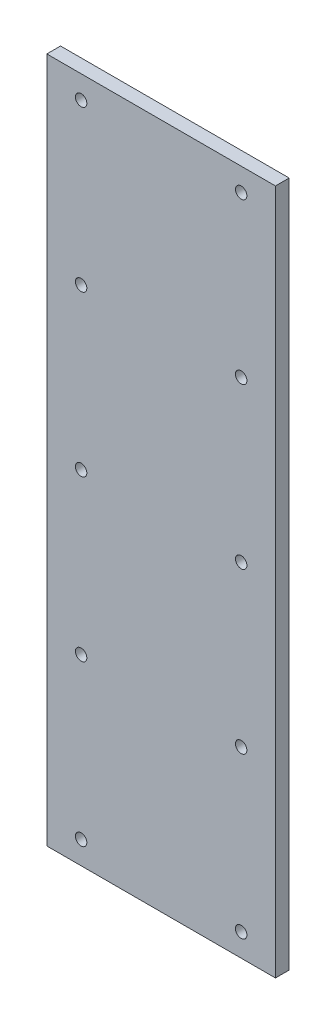
SolidWorks part; units mm, degrees
material "Q235B"
ref_plane "Front Plane" through (0, 0, 0) normal (0, 0, 1) x (1, 0, 0)
ref_plane "Top Plane" through (0, 0, 0) normal (0, 1, 0) x (1, 0, 0)
ref_plane "Right Plane" through (0, 0, 0) normal (1, 0, 0) x (0, 0, -1)
other "Configuration Table"
sketch "Sketch1" plane through (0, 0, 0) normal (0, 0, 1) x (1, 0, 0)
  line L1 (-50, -150) -> (50, -150)
  line L2 (-50, -150) -> (-50, 150)
  line L3 (-50, 150) -> (50, 150)
  line L4 (50, -150) -> (50, 150)
  line L5 (-50, -150) -> (50, 150) construction
  line L6 (-50, 150) -> (50, -150) construction
  circle A0 centre (-35, 0) radius 5.5 construction
  point P0 (0, 0)
  dimension "D1" = 100
  dimension "D2" = 300
  dimension "D3" = 0
  dimension "D4" = 35
extrude "Boss-Extrude1" add sketch "Sketch1" along normal blind 6
hole_wizard "M6 Tapped Hole1" positions "Sketch2" profile "Sketch4" tap size "M6" standard "GB" end condition through all
sketch "Sketch2" plane through (0, 0, 6) normal (0, 0, 1) x (1, 0, 0)
  point P0 (-35, 0)
sketch "Sketch4" plane through (-35, 0, 6) normal (1, 0, 0) x (0, -1, 0)
  line L0 (0, 0) -> (0, 6)
  line L1 (0, 6) -> (2.5, 6)
  line L2 (2.5, 6) -> (2.5, 0)
  line L5 (2.5, 0) -> (0, 0)
  line L11 (0, -6.35) -> (0, 107.95) construction
  dimension "通孔螺纹孔钻头直径" = 5
  dimension "通孔螺纹孔钻头深度" = 6
cosmetic thread "Cosmetic thread 1" parameters "D2"=6
pattern_linear "LPattern1" count 3 spacing 70 along (0, -1, 0) count 2 spacing 70 along (1, 0, 0) of "M6 Tapped Hole1"
pattern_linear "LPattern2" count 3 spacing 70 along (0, 1, 0) of "LPattern1", "M6 Tapped Hole1"
